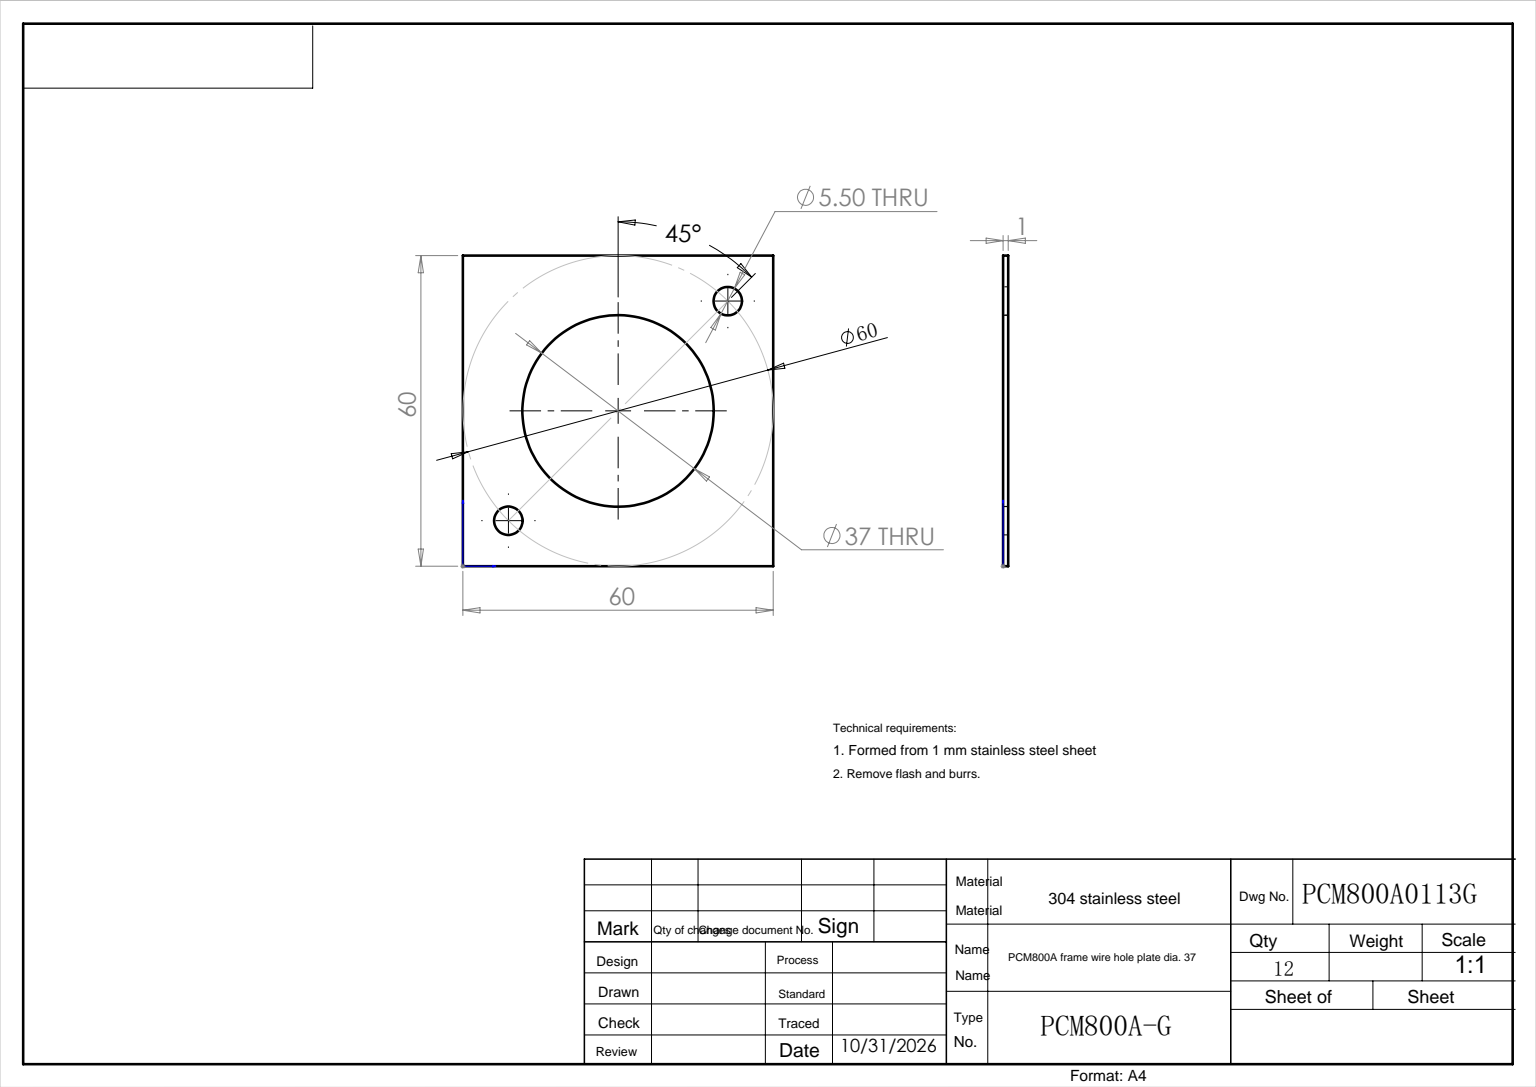
from build123d import *

# Parameters (mm, degrees)
SKETCH_1_W      = 60
SKETCH_1_H      = 60
SKETCH_1_R      = 18.5
SKETCH_1_R_2    = 2.75
EXTRUDE_1_DEPTH = 1


with BuildPart() as part:
    # 草图1 → 凸台-拉伸1 (new body)
    with BuildSketch(Plane.XY):
        with Locations((30, 30)):
            Rectangle(SKETCH_1_W, SKETCH_1_H)
        with Locations((30, 30)):
            Circle(SKETCH_1_R, mode=Mode.SUBTRACT)
        with Locations((8.786796564, 8.786796564)):
            Circle(SKETCH_1_R_2, mode=Mode.SUBTRACT)
        with Locations((51.213203436, 51.213203436)):
            Circle(SKETCH_1_R_2, mode=Mode.SUBTRACT)
    extrude(amount=EXTRUDE_1_DEPTH)


solid = part.part
